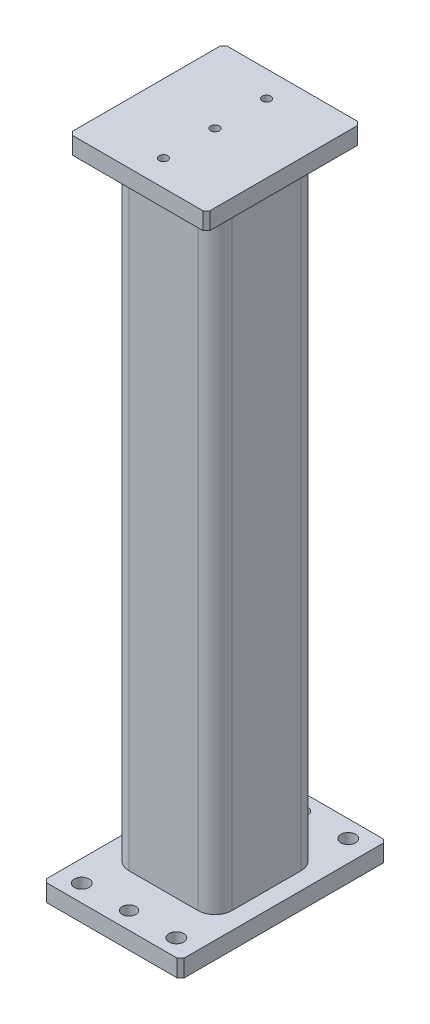
SolidWorks part; units mm, degrees
material "45号钢"
ref_plane "主视基准图" through (0, 0, 0) normal (0, 0, 1) x (1, 0, 0)
ref_plane "上视基准图" through (0, 0, 0) normal (0, 1, 0) x (1, 0, 0)
ref_plane "右视基准图" through (0, 0, 0) normal (1, 0, 0) x (0, 0, -1)
sketch "草图2" plane through (0, 0, 0) normal (0, 0, 1) x (1, 0, 0)
  line L0 (0, 0) -> (0, 359)
  dimension "D1" = 359
other "结构构件1"
ref_plane "基准面1" through (0, 0, 0) normal (0, 1, 0) x (-1, 0, 0)
sketch "Sketch1" plane through (0, 0, 0) normal (0, 1, 0) x (-1, 0, 0)
  line L0 (-20, -25) -> (20, -25)
  line L1 (-25, -20) -> (-25, 20)
  line L2 (20, 25) -> (-20, 25)
  line L3 (25, 20) -> (25, -20)
  line L4 (-20, -30) -> (20, -30)
  line L5 (-30, -20) -> (-30, 20)
  line L6 (20, 30) -> (-20, 30)
  line L7 (30, 20) -> (30, -20)
  arc A0 (30, 20) -> (20, 30) centre (20, 20) ccw
  arc A1 (20, -30) -> (30, -20) centre (20, -20) ccw
  arc A2 (-30, -20) -> (-20, -30) centre (-20, -20) ccw
  arc A3 (-20, 30) -> (-30, 20) centre (-20, 20) ccw
  arc A4 (-20, 25) -> (-25, 20) centre (-20, 20) ccw
  arc A5 (25, 20) -> (20, 25) centre (20, 20) ccw
  arc A6 (20, -25) -> (25, -20) centre (20, -20) ccw
  arc A7 (-25, -20) -> (-20, -25) centre (-20, -20) ccw
  point P0 (-30, 0)
  point P1 (30, 0)
  point P2 (0, 30)
  point P3 (0, -30)
  point P4 (0, 0)
  point P5 (-30, -30)
  point P6 (30, -30)
  point P7 (30, 30)
  point P8 (-30, 30)
  point P33 (0, 0)
  dimension "D1" = 10
  dimension "D2" = 60
  dimension "D3" = 5
sketch "草图4" plane through (0, 0, 0) normal (0, -1, 0) x (1, 0, 0)
  line L0 (0, 0) -> (59.4456, 0) construction
  line L1 (-40, -60) -> (40, -60)
  line L2 (-40, -60) -> (-40, 60)
  line L3 (-40, 60) -> (40, 60)
  line L4 (40, -60) -> (40, 60)
  line L5 (-40, -60) -> (40, 60) construction
  line L6 (-40, 60) -> (40, -60) construction
  point P0 (0, 0)
  dimension "D1" = 80
  dimension "D2" = 120
extrude "凸台-拉伸1" add sketch "草图4" along normal blind 10 separate body
chamfer "倒角1" distance 2 angle 45 4 edges at (40, -5, -60) (-40, -5, -60) (40, -5, 60) (-40, -5, 60)
hole_wizard "Ø8.6 (8.6) 直径孔1" positions "草图6" profile "草图5" hole size "Ø8.6" standard "Ansi Metric"
sketch "草图6" plane through (0, 0, 0) normal (0, 1, 0) x (1, 0, 0)
  line L1 (-27.5, -50) -> (27.5, -50) construction
  line L2 (-27.5, -50) -> (-27.5, 50) construction
  line L3 (-27.5, 50) -> (27.5, 50) construction
  line L4 (27.5, -50) -> (27.5, 50) construction
  line L5 (-27.5, -50) -> (27.5, 50) construction
  line L6 (-27.5, 50) -> (27.5, -50) construction
  line L7 (-38, 60) -> (38, 60) construction
  point P2 (27.5, 50)
  point P83 (-27.5, -50)
  point P84 (-27.5, 50)
  point P85 (27.5, -50)
  dimension "D1" = 10
  dimension "D2" = 55
sketch "草图5" plane through (27.5, 0, -50) normal (1, 0, 0) x (0, 0, 1)
  line L0 (0, 0) -> (0, 18.0926)
  line L1 (0, 18.0926) -> (4.3, 15.61)
  line L2 (4.3, 15.61) -> (4.3, 0)
  line L5 (4.3, 0) -> (0, 0)
  line L10 (0, 18.0926) -> (-4.3, 15.61) construction
  line L11 (0, -6.35) -> (0, 107.95) construction
  dimension "孔直径" = 8.6
  dimension "孔深度" = 15.61
  dimension "导头角度" = 120
hole_wizard "Ø8.0 (8) 直径孔1" positions "草图12" profile "草图11" hole size "Ø8.0" standard "Ansi Metric"
sketch "草图12" plane through (0, 0, 0) normal (0, 1, 0) x (1, 0, 0)
  line L0 (0, 0) -> (-49.5108, 0) construction
  point P0 (0, 50)
  point P2 (0, -50)
  dimension "D1" = 100
sketch "草图11" plane through (0, 0, -50) normal (1, 0, 0) x (0, 0, 1)
  line L0 (0, 0) -> (0, 17.9194)
  line L1 (0, 17.9194) -> (4, 15.61)
  line L2 (4, 15.61) -> (4, 0)
  line L5 (4, 0) -> (0, 0)
  line L10 (0, 17.9194) -> (-4, 15.61) construction
  line L11 (0, -6.35) -> (0, 107.95) construction
  dimension "孔直径" = 8
  dimension "孔深度" = 15.61
  dimension "导头角度" = 120
sketch "草图13" plane through (0, 359, 0) normal (0, 1, 0) x (1, 0, 0)
  line L0 (-40, -58) -> (-40, 58) construction
  line L1 (-40, -45) -> (40, -45)
  line L2 (-40, -45) -> (-40, 45)
  line L3 (-40, 45) -> (40, 45)
  line L4 (40, -45) -> (40, 45)
  line L5 (-40, -45) -> (40, 45) construction
  line L6 (-40, 45) -> (40, -45) construction
  point P0 (0, 0)
  dimension "D1" = 90
extrude "凸台-拉伸2" add sketch "草图13" along normal blind 10 separate body
chamfer "倒角2" distance 2 angle 45 4 edges at (-40, 364, -45) (40, 364, -45) (40, 364, 45) (-40, 364, 45)
hole_wizard "Ø5.0 (5) 直径孔1" positions "草图16" profile "草图15" hole size "Ø5.0" standard "Ansi Metric"
sketch "草图16" plane through (0, 369, 0) normal (0, 1, 0) x (1, 0, 0)
  point P0 (0, 0)
sketch "草图15" plane through (0, 369, 0) normal (1, 0, 0) x (0, 0, 1)
  line L0 (0, 0) -> (0, 17.0534)
  line L1 (0, 17.0534) -> (2.5, 15.61)
  line L2 (2.5, 15.61) -> (2.5, 0)
  line L5 (2.5, 0) -> (0, 0)
  line L10 (0, 17.0534) -> (-2.5, 15.61) construction
  line L11 (0, -6.35) -> (0, 107.95) construction
  dimension "孔直径" = 5
  dimension "孔深度" = 15.61
  dimension "导头角度" = 120
hole_wizard "M6 螺纹孔1" positions "草图18" profile "草图17" tap size "M6" standard "Iso"
sketch "草图18" plane through (0, 369, 0) normal (0, 1, 0) x (1, 0, 0)
  line L0 (0, 0) -> (47.2348, 0) construction
  point P0 (0, 30)
  point P2 (0, -30)
  dimension "D1" = 60
sketch "草图17" plane through (0, 369, -30) normal (1, 0, 0) x (0, 0, 1)
  line L0 (0, 0) -> (0, 18.5022)
  line L1 (0, 18.5022) -> (2.5, 17)
  line L2 (2.5, 17) -> (2.5, 0)
  line L5 (2.5, 0) -> (0, 0)
  line L10 (0, 18.5022) -> (-2.5, 17) construction
  line L11 (0, -6.35) -> (0, 107.95) construction
  dimension "螺纹孔钻头直径" = 5
  dimension "螺纹孔钻头深度" = 17
  dimension "导头角度" = 118
cosmetic thread "孔螺蚊线1"
cosmetic thread "孔螺蚊线2"
